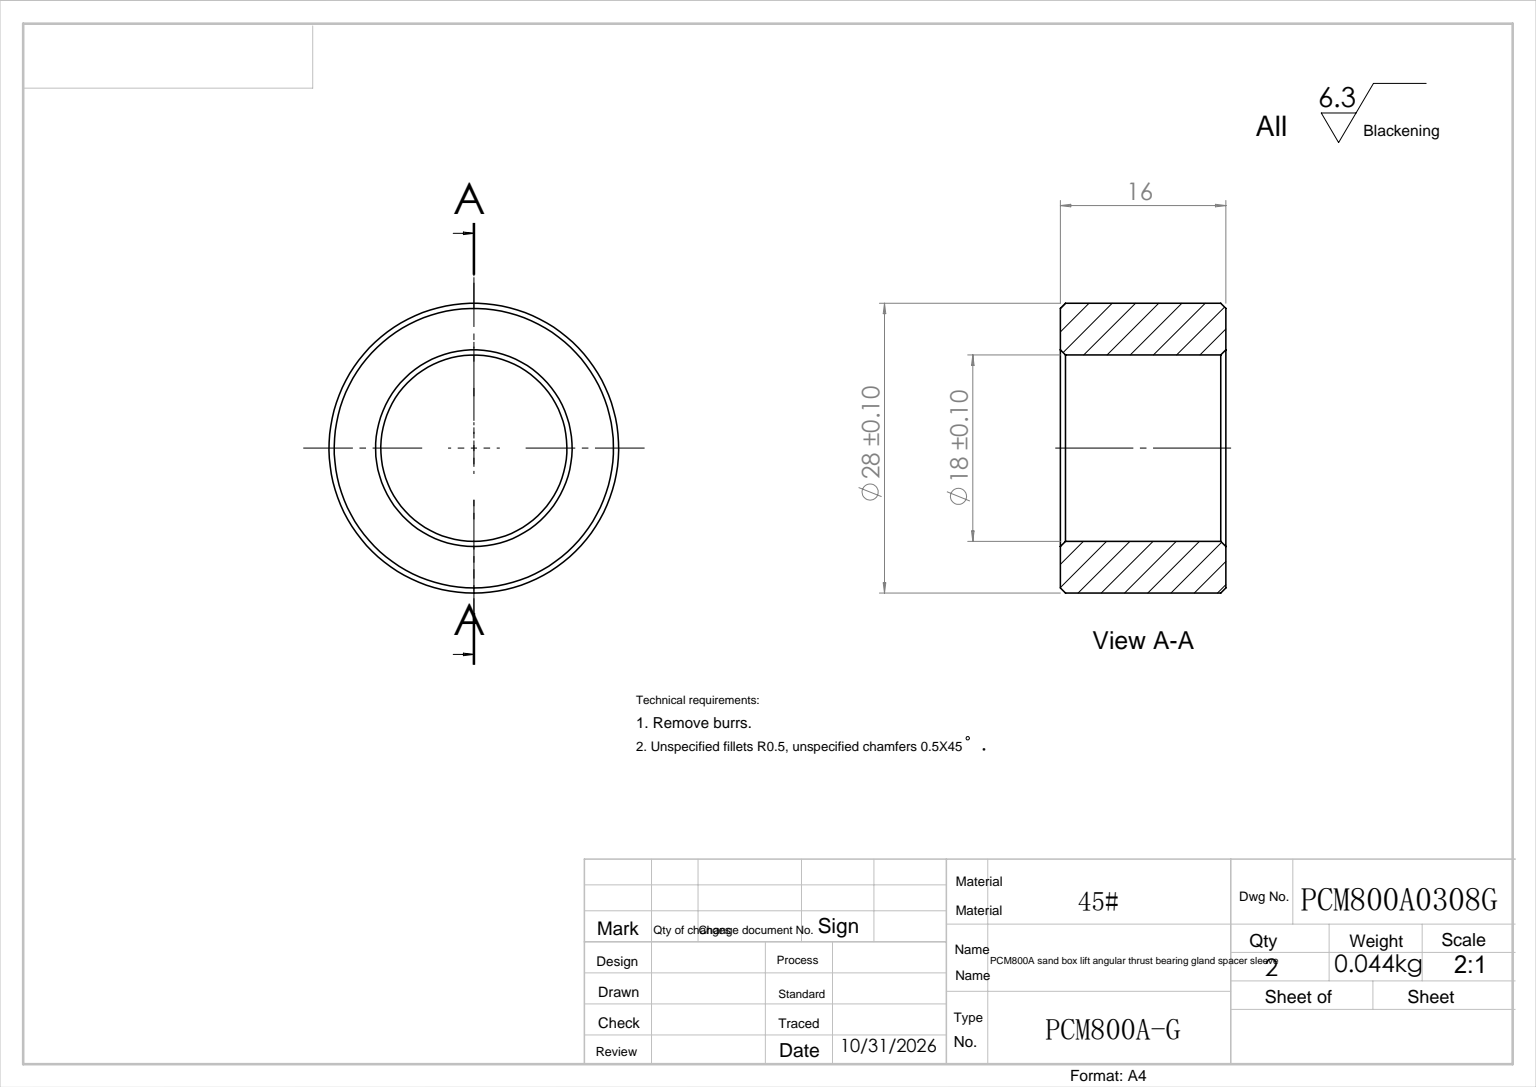
from build123d import *

# Parameters (mm, degrees)
SKETCH_1_R      = 14
SKETCH_1_R_2    = 9
EXTRUDE_1_DEPTH = 16
CHAMFER_1_SIZE  = 0.5


with BuildPart() as part:
    # 草图1 → 拉伸1 (new body)
    with BuildSketch(Plane(origin=(0, 0, 0), x_dir=(1, 0, 0), z_dir=(0, 1, 0))):
        with Locations(Location((0, 0, 0), (0, 0, 270))):
            Circle(SKETCH_1_R)
        with Locations(Location((0, 0, 0), (0, 0, 270))):
            Circle(SKETCH_1_R_2, mode=Mode.SUBTRACT)
    extrude(amount=EXTRUDE_1_DEPTH)

    # 倒角1
    chamfer_1_edges = [part.edges().sort_by_distance(p)[0] for p in [
        (0, 0, -14),
        (0, 16, -14),
        (0, 0, -9),
        (0, 16, -9),
    ]]
    chamfer(chamfer_1_edges, length=CHAMFER_1_SIZE)


solid = part.part
